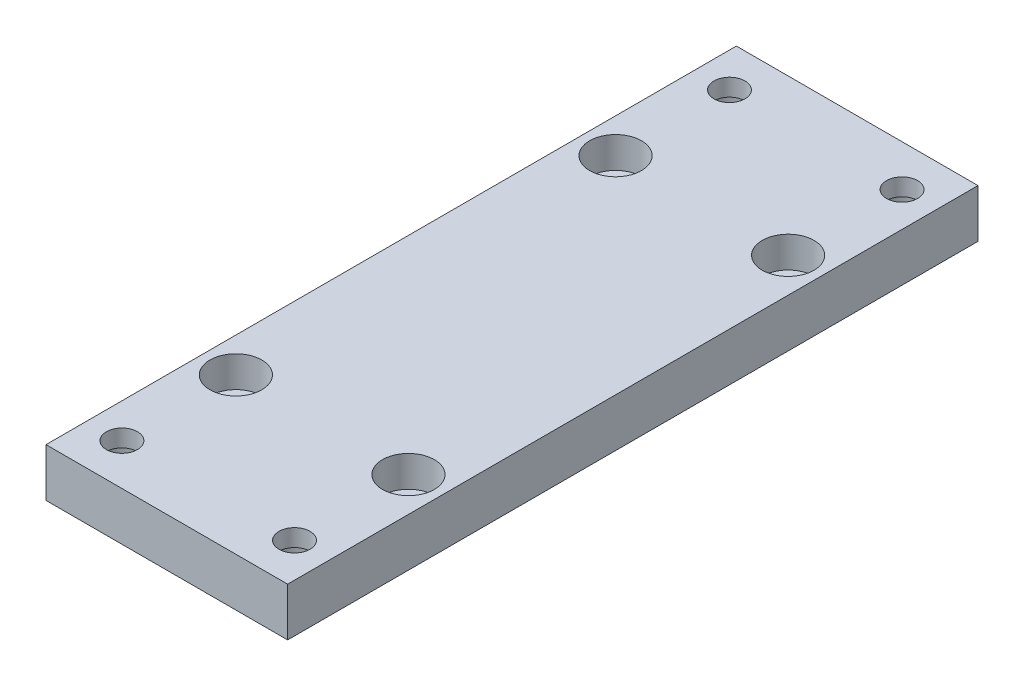
SolidWorks part; units mm, degrees
material "Q235"
ref_plane "Front Plane" through (0, 0, 0) normal (0, 0, 1) x (1, 0, 0)
ref_plane "Top Plane" through (0, 0, 0) normal (0, 1, 0) x (1, 0, 0)
ref_plane "Right Plane" through (0, 0, 0) normal (1, 0, 0) x (0, 0, -1)
sketch "Sketch1" plane through (0, 0, 0) normal (0, 1, 0) x (1, 0, 0)
  line L1 (0, 0) -> (70, 0)
  line L2 (0, 0) -> (0, 200)
  line L3 (0, 200) -> (70, 200)
  line L4 (70, 0) -> (70, 200)
  point P7 (70, 200)
  point P12 (70, 0)
  point P15 (0, 0)
  dimension "D1" = 70
  dimension "D2" = 200
extrude "Boss-Extrude1" add sketch "Sketch1" along normal blind 14
hole_wizard "Hole size (%based on) socket head cap screw type1" positions "Sketch2" profile "Sketch3" counterbore size "M8" standard "GB" end condition through all
sketch "Sketch2" plane through (0, 14, 0) normal (0, 1, 0) x (1, 0, 0)
  line L0 (0, 100) -> (70, 100) construction
  line L1 (0, 200) -> (0, 0) construction
  line L2 (70, 0) -> (70, 200) construction
  line L5 (35, 200) -> (35, 168.287) construction
  line L6 (70, 200) -> (0, 200) construction
  point P0 (10, 155)
  point P2 (60, 155)
  point P4 (60, 45)
  point P6 (10, 45)
  dimension "D1" = 50
  dimension "D2" = 110
sketch "Sketch3" plane through (10, 14, -155) normal (1, 0, 0) x (0, 0, 1)
  line L0 (0, 0) -> (0, 14)
  line L1 (0, 14) -> (4.5, 14)
  line L3 (4.5, 14) -> (4.5, 9)
  line L4 (4.5, 9) -> (7.5, 9)
  line L5 (7.5, 9) -> (7.5, 0)
  line L7 (7.5, 0) -> (0, 0)
  line L11 (0, -6.35) -> (0, 107.95) construction
  dimension "通孔孔直径" = 9
  dimension "通孔孔深度" = 14
  dimension "柱形沉头孔直径" = 15
  dimension "柱形沉头孔深度" = 9
hole_wizard "Hole size (%based on) socket head cap screw type2" positions "Sketch4" profile "Sketch5" counterbore size "M8" standard "GB" end condition through all
sketch "Sketch4" plane through (0, 0, 0) normal (0, -1, 0) x (-1, 0, 0)
  line L0 (-35, 200) -> (-35, 156.1442) construction
  line L1 (-70, 200) -> (0, 200) construction
  line L3 (0, 100) -> (-45.6733, 100) construction
  line L4 (0, 200) -> (0, 0) construction
  point P0 (-60, 188)
  point P2 (-10, 188)
  point P4 (-10, 12)
  point P6 (-60, 12)
  dimension "D1" = 50
  dimension "D2" = 12
sketch "Sketch5" plane through (60, 0, -188) normal (1, 0, 0) x (0, 0, -1)
  line L0 (0, 0) -> (0, 14)
  line L1 (0, 14) -> (4.5, 14)
  line L3 (4.5, 14) -> (4.5, 9)
  line L4 (4.5, 9) -> (7.5, 9)
  line L5 (7.5, 9) -> (7.5, 0)
  line L7 (7.5, 0) -> (0, 0)
  line L11 (0, -6.35) -> (0, 107.95) construction
  dimension "通孔孔直径" = 9
  dimension "通孔孔深度" = 14
  dimension "柱形沉头孔直径" = 15
  dimension "柱形沉头孔深度" = 9
